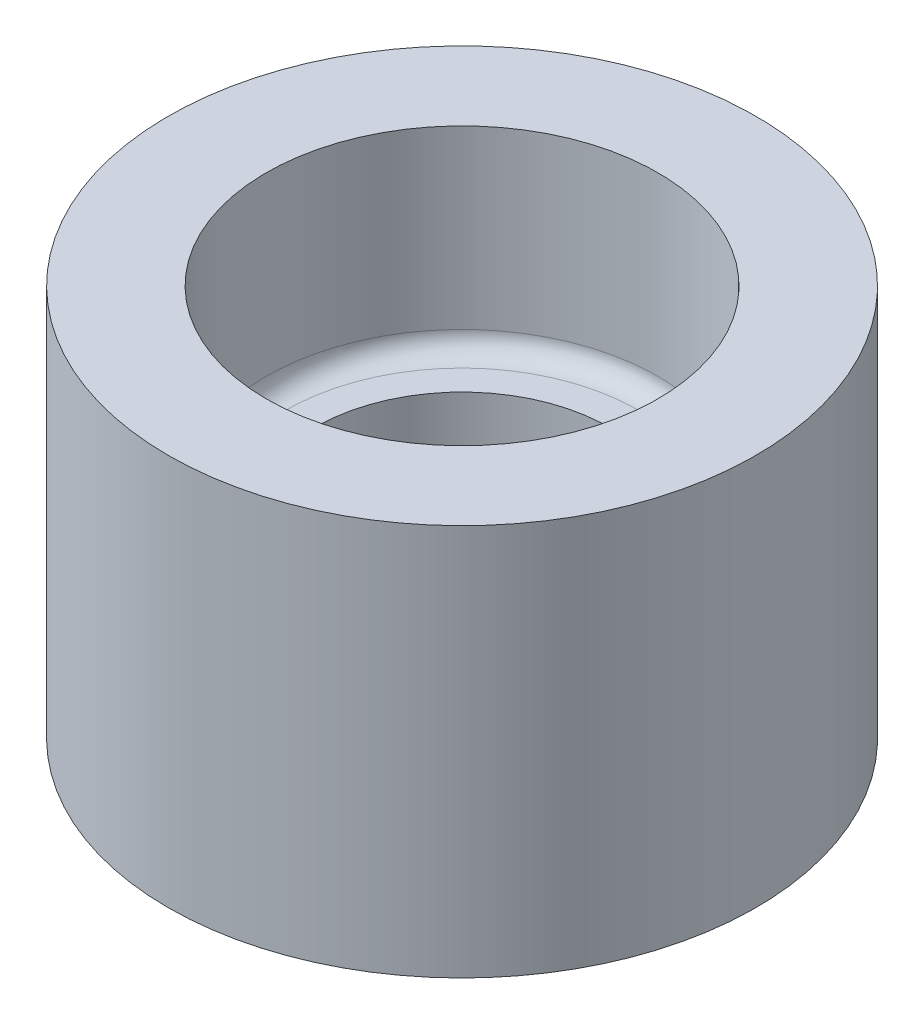
SolidWorks part; units mm, degrees
ref_plane "前视基准面" through (0, 0, 0) normal (0, 0, 1) x (1, 0, 0)
ref_plane "上视基准面" through (0, 0, 0) normal (0, 1, 0) x (1, 0, 0)
ref_plane "右视基准面" through (0, 0, 0) normal (1, 0, 0) x (0, 0, -1)
sketch "草图1" plane through (0, 0, 0) normal (0, 0, 1) x (1, 0, 0)
  line L0 (0, 45.5682) -> (0, -34.8864) construction
  line L1 (15, -20) -> (15, 0)
  line L2 (15, 0) -> (18, 0)
  line L3 (20, 2) -> (20, 20)
  line L4 (20, 20) -> (30, 20)
  line L5 (30, 20) -> (30, -20)
  line L6 (30, -20) -> (15, -20)
  arc A0 (18, 0) -> (20, 2) centre (18, 2) ccw
  dimension "D6" = 2
  dimension "D1" = 15
  dimension "D2" = 15
  dimension "D3" = 20
  dimension "D4" = 5
  dimension "D5" = 40
revolve "旋转1" add sketch "草图1" angle 360 about L0
